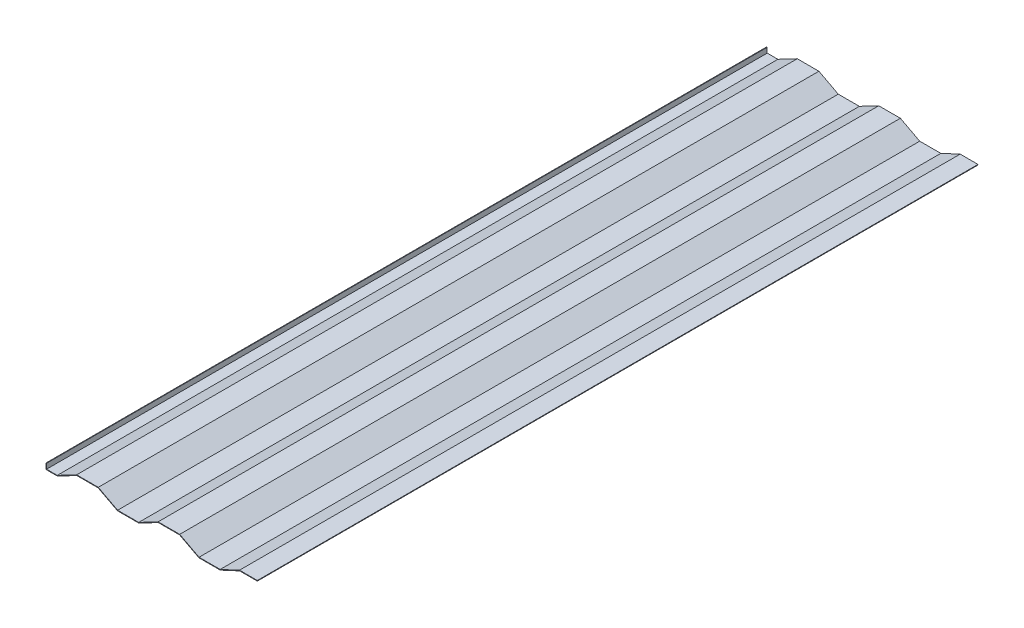
from build123d import *

# Parameters (mm, degrees)
EXTRUDE_THIN1_DEPTH = 2530


with BuildPart() as part:
    # Sketch1 → Extrude-Thin1 (new body)
    with BuildSketch(Plane.XY):
        Polygon((0, 20), (0, 0), (40, 0), (107.973084028, 35.696369631), (182.973084028, 35.696369631), (250.946168056, 0), (325.946168056, 0), (393.919252083, 35.696369631), (468.919252083, 35.696369631), (536.892336111, 0), (611.892336111, 0), (679.865420139, 31.696369631), (742.000000002, 31.696369631), (742.000000002, 33.696369631), (679.422030814, 33.696369631), (611.448946786, 2), (537.385552948, 2), (469.41246892, 37.696369631), (393.426035246, 37.696369631), (325.452951219, 2), (251.439384892, 2), (183.466300865, 37.696369631), (107.479867191, 37.696369631), (39.506783163, 2), (2, 2), (2, 20), align=None)
    extrude(amount=EXTRUDE_THIN1_DEPTH)


solid = part.part
